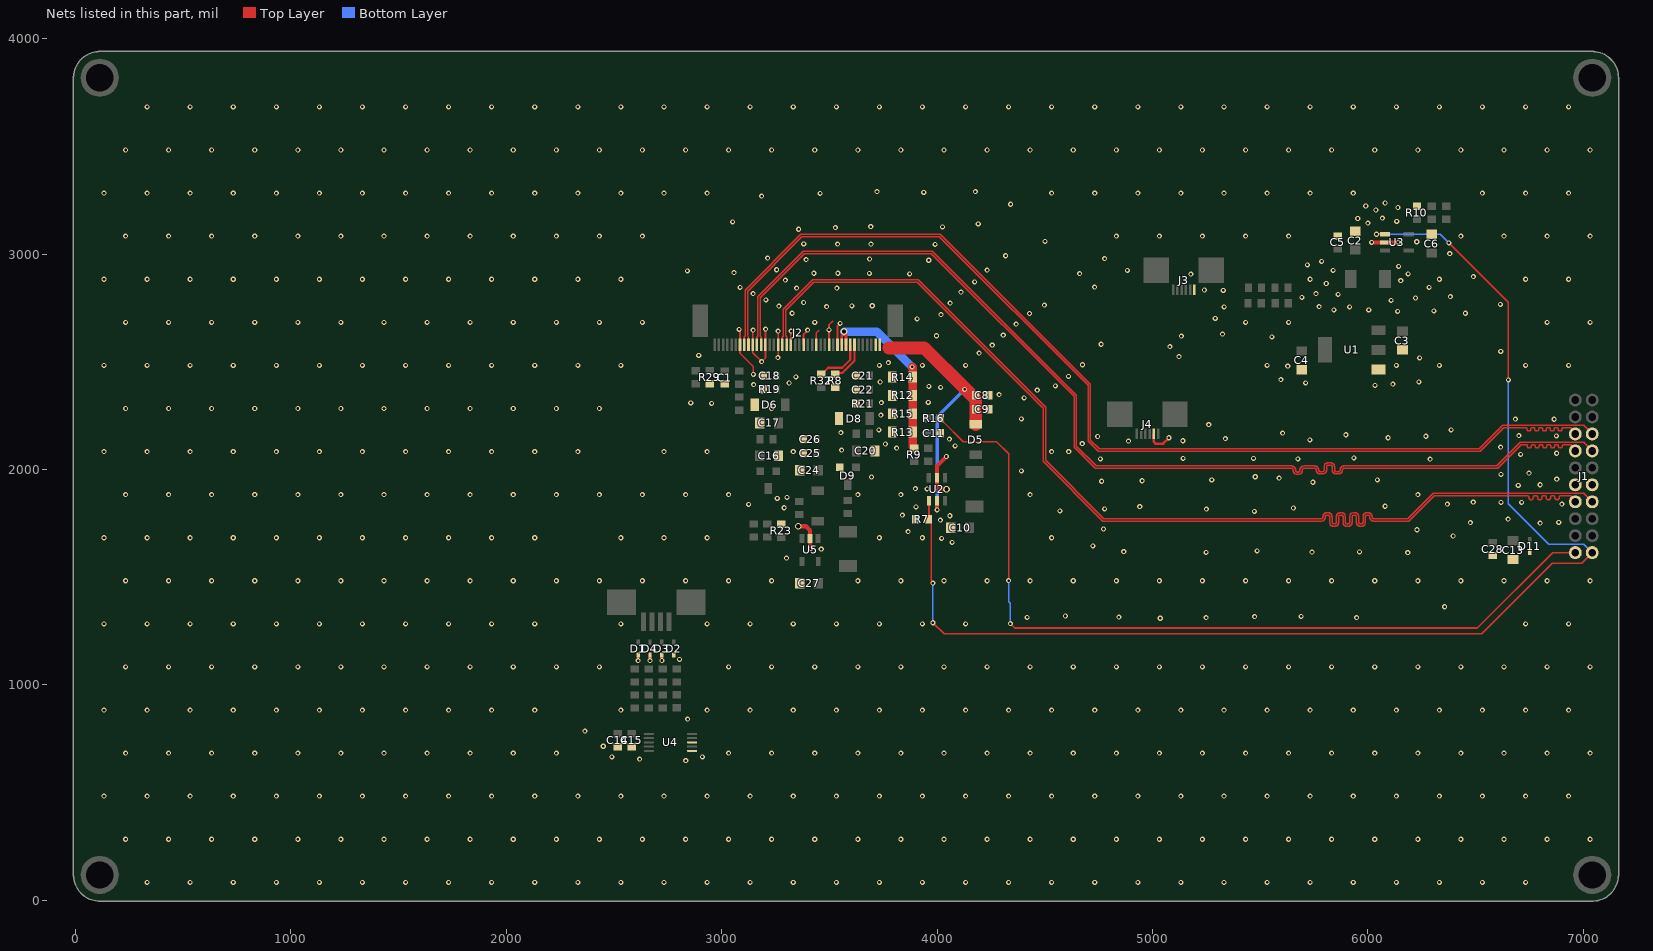
[diagram p0: the nets of this part, all layers, seen from the top]
# Altium PCB MISC82162.PcbDoc (part 2 of 3)
Units mil, origin at the board's own origin, x right, y up, seen from the top; angles counter-clockwise.
Board outline 7173.26 x 3944.91 mil, 2 copper layers (Top Layer, Bottom Layer); 90 components, 54 nets, 272 pads, 794 vias.
Unrouted connection lines stored in the file: 61.

## Via types
v1: diameter 23.62, hole 11.81, Top Layer to Bottom Layer, 779 vias
v2: diameter 32, hole 20, Top Layer to Bottom Layer, 13 vias
v3: diameter 31.5, hole 19.68, Top Layer to Bottom Layer, 2 vias

## Nets (pads, with @x,y where several pads share a name; then routed paths per layer and width w, separated by ;. In a path a pad name is that pad's centre, name@x,y a point inside that pad or via, vN(x,y) a via of type N, cw(c..) or ccw(c..) an arc to the next point about the centre after c; other vN are vias at no path point) (continued)
GND: C1.2 C2.2 C3.2 C4.2 C5.2 C6.2 C8.2 C9.2 C10.2 C11.2 C13.2 C14.2 C15.2 C16.2 C17.2 C18.2 C20.1 C21.2 C22.2 C24.2 C25.2 C26.2 C27.2 C28.1 D1.2 D2.2 D3.2 D4.2 D6.1 D8.2 D9.2 D11.2 J1.11 J1.12 J2.7 J2.10 J2.13 J2.16 J2.19 J2.22 J2.25 J2.28 J2.30 J3.6 J4.5 R7.1 R8.2 R10.2 R12.2 R13.2 R14.2 R15.2 R19.1 R21.1 R23.1 R29.2 U1.1 U2.2 U3.2 U4.6 U4.8 U5.2 | length 1795.5
  Top Layer w8: v1(3081,2650) 3081,2645.77 3084.87,2641.9 J2.7@3084.87,2578.24 3084.87,2540.13 3147,2478 v1(3147,2441) ; v1(3146,2647) 3143.93,2644.93 J2.10@3143.93,2578.24 3144.05,2578.12 3144.05,2541.95 v1(3185,2501) 3202.98,2518.98 J2.13@3202.98,2578.24 3202.98,2651.14 v1(3203.7,2651.86) ; v1(3261,2519) 3262.04,2520.04 J2.16@3262.04,2578.24 v1(3262,2642) v1(3262,2642) ; J2.19@3321.09,2578.24 3321.09,2641.09 v1(3322,2642) ; J2.22@3380.15,2578.24 3380.15,2628.15 v1(3399,2647) ; J2.25@3439.2,2578.24 3439.2,2633.2 3451,2645 ; J2.28@3498.26,2578.24 3498.26,2671.26 3514,2687 ; J2.30@3537.63,2578.24 3537.63,2665.63 v1(3550,2678)
  Top Layer w10: v1(2612,1112) D1.2@2612,1138.47
  Top Layer w12: v1(2667,1112) D4.2@2667,1138.47 ; v1(2722,1113) D3.2@2722,1138.47 ; J4.5@5006.13,2164.85 5006.13,2127.87 5014,2120 5049,2120 v1(5076,2147)
  Top Layer w20: v3(3355,1736) 3391,1736 3410,1717 U5.2@3410,1679.12 3410,1634.98 3413,1631.98 v1(3413,1631) ; v3(4043,1908) 4011.06,1908 3999.34,1919.72 U2.2@3999.34,1961.48 3999.34,2016.34 v1(4043,2060) ; v1(6017,3054) U3.2@6079.39,3054.03 ; U3.2@6079.39,3054.03 v1(6141,3054)
  other v1: 332,83 532,83 732,83 932,83 1132,83 1332,83 1532,83 1732,83 1932,83 2132,83 2332,83 2532,83 2732,83 2932,83 3132,83 3332,83 3532,83 3732,83 3932,83 4132,83 4332,83 4532,83 4732,83 4932,83 5132,83 5332,83 5532,83 5732,83 5932,83 6132,83 6332,83 6532,83 6732,83 232,283 432,283 632,283 832,283 1032,283 1232,283 1432,283 1632,283 1832,283 2032,283 2232,283 2432,283 2632,283 2832,283 3032,283 3232,283 3432,283 3632,283 3832,283 4032,283 4232,283 4432,283 4632,283 4832,283 5032,283 5232,283 5432,283 5632,283 5832,283 6032,283 6232,283 6432,283 6632,283 6832,283 7032,283 132,483 332,483 532,483 732,483 932,483 1132,483 1332,483 1532,483 1732,483 1932,483 2132,483 2332,483 2532,483 2732,483 2932,483 3132,483 3332,483 3532,483 3732,483 3932,483 4132,483 4332,483 4532,483 4732,483 4932,483 5132,483 5332,483 5532,483 5732,483 5932,483 6132,483 6332,483 6532,483 6732,483 6932,483 2833.13,647.92 2618.85,655.14 2490,665 2910,665 232,683 432,683 632,683 832,683 1032,683 1232,683 1432,683 1632,683 1832,683 2032,683 2232,683 3032,683 3232,683 3432,683 3632,683 3832,683 4032,683 4232,683 4432,683 4632,683 4832,683 5032,683 5232,683 5432,683 5632,683 5832,683 6032,683 6232,683 6432,683 6632,683 6832,683 7032,683 2450,715 2365,785 2842.07,840.37 132,883 332,883 532,883 732,883 932,883 1132,883 1332,883 1532,883 1732,883 1932,883 2132,883 2532,883 2932,883 3132,883 3332,883 3532,883 3732,883 3932,883 4132,883 4332,883 4532,883 4732,883 4932,883 5132,883 5332,883 5532,883 5732,883 5932,883 6132,883 6332,883 6532,883 6732,883 6932,883 232,1083 432,1083 632,1083 832,1083 1032,1083 1232,1083 1432,1083 1632,1083 1832,1083 2032,1083 2232,1083 2432,1083 3032,1083 3232,1083 3432,1083 3632,1083 3832,1083 4032,1083 4232,1083 4432,1083 4632,1083 4832,1083 5032,1083 5232,1083 5432,1083 5632,1083 5832,1083 6032,1083 6232,1083 6432,1083 6632,1083 6832,1083 7032,1083 2804,1118 132,1283 332,1283 532,1283 732,1283 932,1283 1132,1283 1332,1283 1532,1283 1732,1283 1932,1283 2132,1283 2532,1283 2932,1283 3132,1283 3332,1283 3532,1283 3732,1283 3932,1283 4132,1283 6732,1283 6932,1283 5036,1309 5248.61,1311.66 5948,1312 4418,1313 4844,1314 5474,1317 5689.95,1317.55 4595.37,1319.57 6355.94,1362.48 232,1483 432,1483 632,1483 832,1483 1032,1483 1232,1483 1432,1483 1632,1483 1832,1483 2032,1483 2232,1483 2432,1483 2632,1483 2832,1483 3032,1483 3232,1483 3632,1483 3832,1483 4032,1483 4232,1483 4432,1483 4632,1483 4832,1483 5032,1483 5232,1483 5432,1483 5632,1483 5832,1483 6032,1483 6232,1483 6432,1483 6632,1483 6832,1483 7032,1483 3300.7,1588.65 6185,1614 5248.62,1615.21 5740.6,1616.55 5961,1617 4866.54,1618.84 5486,1622 3462,1630 4723,1645 4070,1661 4021,1680 132,1683 332,1683 532,1683 732,1683 932,1683 1132,1683 1332,1683 1532,1683 1732,1683 1932,1683 2132,1683 2532,1683 2732,1683 2932,1683 3732,1683 3932,1683 4532,1683 6396,1691 3865.22,1711.62 6228,1720 4772.53,1723.45 6800,1751 6475.87,1752.94 6886,1754 4015,1765 6651,1769 4059,1785 3838.91,1787.51 5473,1805 4569.73,1807.59 5250.06,1815.91 4777.4,1816.99 5654,1821 3290,1822 3902,1826 4941,1827 6080,1829 3124.89,1837.71 6369,1839 6901,1839 6618,1847 6714,1847 6489,1848 3257.95,1865.44 3303.13,1870.12 232,1883 432,1883 632,1883 832,1883 1032,1883 1232,1883 1432,1883 1632,1883 1832,1883 2032,1883 2232,1883 2432,1883 2632,1883 2832,1883 3032,1883 3632,1883 3832,1883 4432,1883 6232,1883 3954,1910 3899,1911 6698,1926 6800,1929 5744.95,1940.52 4764,1945 4952.09,1947.57 5275,1951.73 6043.88,1951.61 6877,1955 5587.61,1959.59 3695.4,1964.97 5477,1966 6618,1977 6748,1983 4391,1993 6289,2048 4758.45,2049.05 5675,2049 5142,2051 5469,2051 5935,2054 6709,2070 6876,2075 132,2083 332,2083 532,2083 732,2083 932,2083 1132,2083 1332,2083 1532,2083 1732,2083 1932,2083 2132,2083 2332,2083 2732,2083 2932,2083 3332,2083 4532,2083 4611,2083 3556.73,2089.96 3812,2099 6616,2104 4084,2109 3760,2118 4674,2120 4888.49,2131.16 5141,2133 5731,2137 4057,2141 5338,2143 6093.93,2147.08 4745,2153 6269,2154 6875,2156 6701,2157 5898,2161 5604,2169 3553.45,2171.18 3729.32,2183.49 6386.63,2183.84 5261,2208 6865,2233 6685,2234 4391,2235 3739,2252 232,2283 432,2283 632,2283 832,2283 1032,2283 1232,2283 1432,2283 1632,2283 1832,2283 2032,2283 2232,2283 2432,2283 3232,2283 2953,2307 2856.26,2308.9 3741.58,2310.22 3958.86,2310.95 4404,2332 4288,2347 4465,2368 4016.17,2380.6 3962,2386 4549,2388 6033,2390 3148,2394 6116.3,2396.25 3312.51,2401.24 5711,2402 3735,2406 6236.99,2406.13 5595.77,2417.43 3344.1,2429.47 4610,2432 5627.97,2479.62 132,2483 332,2483 532,2483 732,2483 932,2483 1132,2483 1332,2483 1532,2483 1732,2483 1932,2483 2132,2483 2332,2483 2532,2483 3732,2483 3932,2483 4132,2483 5532,2483 6132,2483 6332,2483 6732,2483 6932,2483 4675,2486 3774,2496 6239.81,2517.65 5123,2524 2893.23,2529.51 4195,2540 6617,2548 5081,2570 4256,2577 4761.52,2581.24 5553.87,2615.24 5134,2619 3997.15,2620.52 4307,2624 5325,2628 3498,2648 4367,2675 232,2683 432,2683 632,2683 832,2683 1032,2683 1232,2683 1432,2683 1632,2683 1832,2683 2032,2683 2232,2683 2432,2683 2632,2683 3432,2683 5432,2683 5632,2683 6832,2683 7032,2683 3907,2699 5291.38,2700.88 4018,2719 4429,2724 3327,2725 6453,2725 6138,2734 6306.08,2736.13 5842.15,2740.37 6004.14,2740.37 5332.33,2754.87 5915,2755 3487,2756 5773.45,2755.63 3265,2758 3604,2759 3699,2760 4498,2763 6615,2766 4060,2772 3380,2775 6108,2785 3205,2787 6221,2796 5693.72,2798.89 6383,2802 5861.66,2812.46 3146,2816 5759.03,2816.7 4111,2823 5328.29,2830.92 5241,2833 3348,2842 3535,2842 3085,2845 4731.5,2846.16 6284.03,2845.53 5806.53,2863.35 4174,2871 6152.57,2876.92 3296,2879 132,2883 332,2883 532,2883 732,2883 932,2883 1132,2883 1332,2883 1532,2883 1732,2883 1932,2883 2132,2883 2332,2883 2532,2883 5732,2883 6332,2883 6732,2883 6932,2883 6490,2895 5178,2907 3872.33,2908 6187,2908 4661.36,2908.75 3686,2910 3428,2911 3539,2911 3057,2914 2840.2,2921.39 4883.66,2923.85 5838.76,2924.41 4232,2925 3255,2927 6143,2943 5719.17,2949.85 5785.32,2965.97 3961,2971 3392,2974 3687,2977 4777.9,2978.89 3213,2981 4318,2992 6380,3002 3991,3045 3538,3046 3693,3046 3381,3047 6227,3057 4501,3059 232,3083 432,3083 632,3083 832,3083 1032,3083 1232,3083 1432,3083 1632,3083 1832,3083 2032,3083 2232,3083 2432,3083 2632,3083 4832,3083 5032,3083 5232,3083 5432,3083 5632,3083 6432,3083 6632,3083 6832,3083 7032,3083 3357,3115 3528,3123 4025,3126 3691.97,3126.97 4191,3140 6000,3144 3050.2,3149.2 6134,3152 5953,3165 6067,3167 6037.22,3204.5 6139.7,3216.1 5990,3223 4341,3231 6080,3237 3185.55,3268.76 3457,3282 132,3283 332,3283 532,3283 732,3283 932,3283 1132,3283 1332,3283 1532,3283 1732,3283 1932,3283 2132,3283 2332,3283 2532,3283 2732,3283 2932,3283 4532,3283 4732,3283 4932,3283 5132,3283 5332,3283 5532,3283 5732,3283 5932,3283 6532,3283 6732,3283 6932,3283 3938,3286 3721,3290 4177.9,3289.68 232,3483 432,3483 632,3483 832,3483 1032,3483 1232,3483 1432,3483 1632,3483 1832,3483 2032,3483 2232,3483 2432,3483 2632,3483 2832,3483 3032,3483 3232,3483 3432,3483 3632,3483 3832,3483 4032,3483 4232,3483 4432,3483 4632,3483 4832,3483 5032,3483 5232,3483 5432,3483 5632,3483 5832,3483 6032,3483 6232,3483 6432,3483 6632,3483 6832,3483 7032,3483 332,3683 532,3683 732,3683 932,3683 1132,3683 1332,3683 1532,3683 1732,3683 1932,3683 2132,3683 2332,3683 2532,3683 2732,3683 2932,3683 3132,3683 3332,3683 3532,3683 3732,3683 3932,3683 4132,3683 4332,3683 4532,3683 4732,3683 4932,3683 5132,3683 5332,3683 5532,3683 5732,3683 5932,3683 6132,3683 6332,3683 6532,3683 6732,3683 6932,3683
LCD-BL-EN: J1.20 R7.2 U2.4 U3.1 | length 6018.5
  Top Layer w6: R7.2@3959.66,1768.33 3973.39,1754.6 3973.39,1483.38 3980,1476.77 v1(3980,1472) ; v1(3980,1288) 4032,1236 6528,1236 6856,1564 6991.9,1564 J1.20@7041.57,1613.67 ; v1(6040,3092) 6078.82,3092 U3.1@6079.39,3091.43 ; v1(6376,3052) 6652,2776 v1(6652,2416)
  Top Layer w8: R7.2@3959.66,1768.33 3962.14,1770.81 U2.4@3962.14,1855.18
  Bottom Layer w6: v1(3980,1288) v1(3980,1472) ; v1(6040,3092) 6336,3092 v1(6376,3052) ; v1(6652,2416) 6652,1840 6840,1652 6904,1652 6904.56,1652.56 7002.68,1652.56 J1.20@7041.57,1613.67
LCD-PWM: J1.19 R16.2 | length 3952.3
  Top Layer w8: R16.2@4014.66,2235.38 4027.39,2222.65 4122.04,2128 4276,2128 4332,2072 v1(4332,1484) ; v1(4340,1284) 4360,1264 6508,1264 6857.65,1613.65 J1.19@6962.83,1613.65
  Bottom Layer w8: v1(4332,1484) 4332,1386.51 4340,1378.51 v1(4340,1284)
LCD_LR: J2.33 R32.2 | length 231.8
  Top Layer w10: R32.2@3461.99,2442.22 3464.94,2442.22 3494.72,2472 3560,2472 3596.68,2508.68 J2.33@3596.68,2578.24
LCD_UD: J2.34 R8.1 | length 189
  Top Layer w10: R8.1@3526.99,2442.22 3532.77,2448 3560,2448 3616.37,2504.37 J2.34@3616.37,2578.24
LED9.3V: C8.1 C9.1 D5.2 J2.39 J2.40 U2.5 | length 1274.4
  Top Layer w16: U2.5@3999.34,1855.18 3999.67,1854.85 3999.67,1812.33 v1(4000,1812)
  Top Layer w60: 3776,2564 3940,2564 4130,2374 4179.34,2324.66 D5.2@4179.34,2209.2
  Bottom Layer w16: v1(4000,1812) 4000,2244 v1(4128,2372)
LED-: J2.31 J2.32 R9.1 R12.1 R13.1 R14.1 R15.1 | length 891.8
  Top Layer w12: J2.31@3557.31,2578.24 3557.31,2623.9 v2@3568,2634.59 ; v2(3568,2640) v2@3568,2634.59 ; J2.32@3577,2578.24 3577,2625.59 v2@3568,2634.59
  Top Layer w40: v1(3884,2476) 3886.62,2473.38 R14.1@3886.62,2428.64 R12.1@3886.62,2343.64 R15.1@3886.62,2258.64 R13.1@3886.62,2173.64 3886.62,2106.37 R9.1@3894.34,2098.65
  Bottom Layer w40: v2(3568,2640) 3720,2640 v1(3884,2476)
LVDS0-CLKN: J1.14 J2.17 | length 4925.1
  Top Layer w6: J2.17@3281.72,2578.24 3281.72,2614.72 3286.07,2619.07 3286.07,2742.62 3423.44,2880 3911.56,2880 4504,2287.56 4504,2041.56 4774.56,1771 5775,1771 5783.5,1771 ccw(c5783.5,1779) 5791.5,1779 5791.5,1780.25 cw(c5810.5,1780.25) 5810.5,1799.25 5814.5,1799.25 cw(c5814.5,1780.25) 5833.5,1780.25 5833.5,1754.99 ccw(c5841.5,1754.99) 5841.5,1746.99 5845.5,1746.99 ccw(c5845.5,1754.99) 5853.5,1754.99 5853.5,1780.25 cw(c5872.5,1780.25) 5872.5,1799.25 5876.5,1799.25 cw(c5876.5,1780.25) 5895.5,1780.25 5895.5,1754.99 ccw(c5903.5,1754.99) 5903.5,1746.99 5907.5,1746.99 ccw(c5907.5,1754.99) 5915.5,1754.99 5915.5,1780.25 cw(c5934.5,1780.25) 5934.5,1799.25 5938.5,1799.25 cw(c5938.5,1780.25) 5957.5,1780.25 5957.5,1754.99 ccw(c5965.5,1754.99) 5965.5,1746.99 5969.5,1746.99 ccw(c5969.5,1754.99) 5977.5,1754.99 5977.5,1780.25 cw(c5996.5,1780.25) 5996.5,1799.25 6000.5,1799.25 cw(c6000.5,1780.25) 6019.5,1780.25 6019.5,1779 ccw(c6027.5,1779) 6027.5,1771 6068.03,1771 6185.44,1771 6304.19,1889.74 7001.71,1889.74 J1.14@7041.57,1849.89
LVDS0-CLKP: J1.13 J2.18 | length 4904.3
  Top Layer w6: J2.18@3302,2597.49 3302,2615 3297.07,2619.93 3297.07,2738.07 3428,2869 3907,2869 4493,2283 4493,2037 4770,1760 5775,1760 5783.5,1760 ccw(c5783.5,1779) 5802.5,1779 5802.5,1780.25 cw(c5810.5,1780.25) 5810.5,1788.25 5814.5,1788.25 cw(c5814.5,1780.25) 5822.5,1780.25 5822.5,1754.99 ccw(c5841.5,1754.99) 5841.5,1735.99 5845.5,1735.99 ccw(c5845.5,1754.99) 5864.5,1754.99 5864.5,1780.25 cw(c5872.5,1780.25) 5872.5,1788.25 5876.5,1788.25 cw(c5876.5,1780.25) 5884.5,1780.25 5884.5,1754.99 ccw(c5903.5,1754.99) 5903.5,1735.99 5907.5,1735.99 ccw(c5907.5,1754.99) 5926.5,1754.99 5926.5,1780.25 cw(c5934.5,1780.25) 5934.5,1788.25 5938.5,1788.25 cw(c5938.5,1780.25) 5946.5,1780.25 5946.5,1754.99 ccw(c5965.5,1754.99) 5965.5,1735.99 5969.5,1735.99 ccw(c5969.5,1754.99) 5988.5,1754.99 5988.5,1780.25 cw(c5996.5,1780.25) 5996.5,1788.25 6000.5,1788.25 cw(c6000.5,1780.25) 6008.5,1780.25 6008.5,1779 ccw(c6027.5,1779) 6027.5,1760 6068.03,1760 6190,1760 6308.74,1878.74 6717,1878.74 6740,1878.74 cw(c6740,1870.74) 6748,1870.74 6748,1867.97 ccw(c6756,1867.97) 6756,1859.97 6760,1859.97 ccw(c6760,1867.97) 6768,1867.97 6768,1870.74 cw(c6776,1870.74) 6776,1878.74 6780,1878.74 cw(c6780,1870.74) 6788,1870.74 6788,1867.97 ccw(c6796,1867.97) 6796,1859.97 6800,1859.97 ccw(c6800,1867.97) 6808,1867.97 6808,1870.74 cw(c6816,1870.74) 6816,1878.74 6820,1878.74 cw(c6820,1870.74) 6828,1870.74 6828,1867.97 ccw(c6836,1867.97) 6836,1859.97 6840,1859.97 ccw(c6840,1867.97) 6848,1867.97 6848,1870.74 cw(c6856,1870.74) 6856,1878.74 6860,1878.74 cw(c6860,1870.74) 6868,1870.74 6868,1867.97 ccw(c6876,1867.97) 6876,1859.97 6880,1859.97 ccw(c6880,1867.97) 6888,1867.97 6888,1870.74 cw(c6896,1870.74) 6896,1878.74 6915,1878.74 6941.54,1878.74 6962.83,1857.46 J1.13@6962.83,1849.85
LVDS0-D0N: J1.6 J2.8 | length 4921.6
  Top Layer w6: J2.8@3104.56,2578.24 3104.56,2616.66 3108.9,2621 3108.9,2832.9 3368,3092 4014.56,3092 4712,2394.56 4712,2136.56 4752.56,2096 6516.44,2096 6625.09,2204.64 6711.91,2204.64 6810.71,2204.64 7001.77,2204.64 J1.6@7041.57,2164.85
LVDS0-D0P: J1.5 J2.9 | length 4919.7
  Top Layer w6: J2.9@3124.24,2578.24 3124.24,2617.66 3119.9,2622 3119.9,2828.35 3372.56,3081 4010,3081 4701,2390 4701,2132 4748,2085 6521,2085 6629.64,2193.64 6711.91,2193.64 6732.91,2193.64 cw(c6732.91,2187.64) 6738.91,2187.64 6738.91,2184.63 ccw(c6743.41,2184.63) 6743.41,2180.13 6752.41,2180.13 ccw(c6752.41,2184.63) 6756.91,2184.63 6756.91,2189.14 cw(c6761.41,2189.14) 6761.41,2193.64 6770.41,2193.64 cw(c6770.41,2189.14) 6774.91,2189.14 6774.91,2184.63 ccw(c6779.41,2184.63) 6779.41,2180.13 6788.41,2180.13 ccw(c6788.41,2184.63) 6792.91,2184.63 6792.91,2189.14 cw(c6797.41,2189.14) 6797.41,2193.64 6806.41,2193.64 cw(c6806.41,2189.14) 6810.91,2189.14 6810.91,2184.63 ccw(c6815.41,2184.63) 6815.41,2180.13 6824.41,2180.13 ccw(c6824.41,2184.63) 6828.91,2184.63 6828.91,2189.14 cw(c6833.41,2189.14) 6833.41,2193.64 6842.41,2193.64 cw(c6842.41,2189.14) 6846.91,2189.14 6846.91,2184.63 ccw(c6851.41,2184.63) 6851.41,2180.13 6860.41,2180.13 ccw(c6860.41,2184.63) 6864.91,2184.63 6864.91,2189.14 cw(c6869.41,2189.14) 6869.41,2193.64 6878.41,2193.64 cw(c6878.41,2189.14) 6882.91,2189.14 6882.91,2184.63 ccw(c6887.41,2184.63) 6887.41,2180.13 6896.41,2180.13 ccw(c6896.41,2184.63) 6900.91,2184.63 6900.91,2187.64 cw(c6906.91,2187.64) 6906.91,2193.64 6920.18,2193.64 6941.44,2193.64 6962.83,2172.26 J1.5@6962.83,2164.85
LVDS0-D1N: J1.8 J2.11 | length 4904
  Top Layer w6: J2.11@3163,2597.51 3163,2614 3167.96,2618.96 3167.96,2801.96 3379,3013 3977.56,3013 4647,2343.56 4647,2107.56 4738.56,2016 5577,2016 5645.5,2016 cw(c5645.5,1997) 5664.5,1997 5664.5,1995.91 ccw(c5672.5,1995.91) 5672.5,1987.91 5676.5,1987.91 ccw(c5676.5,1995.91) 5684.5,1995.91 5684.5,1997 cw(c5703.5,1997) 5703.5,2016 5712,2016 5753.63,2016 cw(c5753.63,1998.5) 5771.13,1998.5 5771.13,1996.82 ccw(c5777.63,1996.82) 5777.63,1990.32 5790.63,1990.32 ccw(c5790.63,1996.82) 5797.13,1996.82 5797.13,2012.86 cw(c5814.63,2012.86) 5814.63,2030.36 5827.63,2030.36 cw(c5827.63,2012.86) 5845.13,2012.86 5845.13,1996.82 ccw(c5851.63,1996.82) 5851.63,1990.32 5864.63,1990.32 ccw(c5864.63,1996.82) 5871.13,1996.82 5871.13,1998.5 cw(c5888.63,1998.5) 5888.63,2016 6598.44,2016 6708.39,2125.94 7001.73,2125.94 J1.8@7041.57,2086.11
LVDS0-D1P: J1.7 J2.12 | length 4920
  Top Layer w6: J2.12@3183.3,2578.24 3183.3,2614.7 3178.96,2619.04 3178.96,2797.4 3383.56,3002 3973,3002 4636,2339 4636,2103 4734,2005 5645.5,2005 cw(c5645.5,1997) 5653.5,1997 5653.5,1995.91 ccw(c5672.5,1995.91) 5672.5,1976.91 5676.5,1976.91 ccw(c5676.5,1995.91) 5695.5,1995.91 5695.5,1997 cw(c5703.5,1997) 5703.5,2005 5753.63,2005 cw(c5753.63,1998.5) 5760.13,1998.5 5760.13,1996.82 ccw(c5777.63,1996.82) 5777.63,1979.32 5790.63,1979.32 ccw(c5790.63,1996.82) 5808.13,1996.82 5808.13,2012.86 cw(c5814.63,2012.86) 5814.63,2019.36 5827.63,2019.36 cw(c5827.63,2012.86) 5834.13,2012.86 5834.13,1996.82 ccw(c5851.63,1996.82) 5851.63,1979.32 5864.63,1979.32 ccw(c5864.63,1996.82) 5882.13,1996.82 5882.13,1998.5 cw(c5888.63,1998.5) 5888.63,2005 6603,2005 6712.94,2114.94 6713.66,2114.94 6734.66,2114.94 cw(c6734.66,2108.94) 6740.66,2108.94 6740.66,2106.24 ccw(c6746.06,2106.24) 6746.06,2100.84 6753.26,2100.84 ccw(c6753.26,2106.24) 6758.66,2106.24 6758.66,2109.54 cw(c6764.06,2109.54) 6764.06,2114.94 6771.26,2114.94 cw(c6771.26,2109.54) 6776.66,2109.54 6776.66,2106.24 ccw(c6782.06,2106.24) 6782.06,2100.84 6789.26,2100.84 ccw(c6789.26,2106.24) 6794.66,2106.24 6794.66,2109.54 cw(c6800.06,2109.54) 6800.06,2114.94 6807.26,2114.94 cw(c6807.26,2109.54) 6812.66,2109.54 6812.66,2106.24 ccw(c6818.06,2106.24) 6818.06,2100.84 6825.26,2100.84 ccw(c6825.26,2106.24) 6830.66,2106.24 6830.66,2109.54 cw(c6836.06,2109.54) 6836.06,2114.94 6843.26,2114.94 cw(c6843.26,2109.54) 6848.66,2109.54 6848.66,2106.24 ccw(c6854.06,2106.24) 6854.06,2100.84 6861.26,2100.84 ccw(c6861.26,2106.24) 6866.66,2106.24 6866.66,2109.54 cw(c6872.06,2109.54) 6872.06,2114.94 6879.26,2114.94 cw(c6879.26,2109.54) 6884.66,2109.54 6884.66,2106.24 ccw(c6890.06,2106.24) 6890.06,2100.84 6897.26,2100.84 ccw(c6897.26,2106.24) 6902.66,2106.24 6902.66,2108.94 cw(c6908.66,2108.94) 6908.66,2114.94 6921.43,2114.94 6941.44,2114.94 6962.83,2093.56 J1.7@6962.83,2086.15